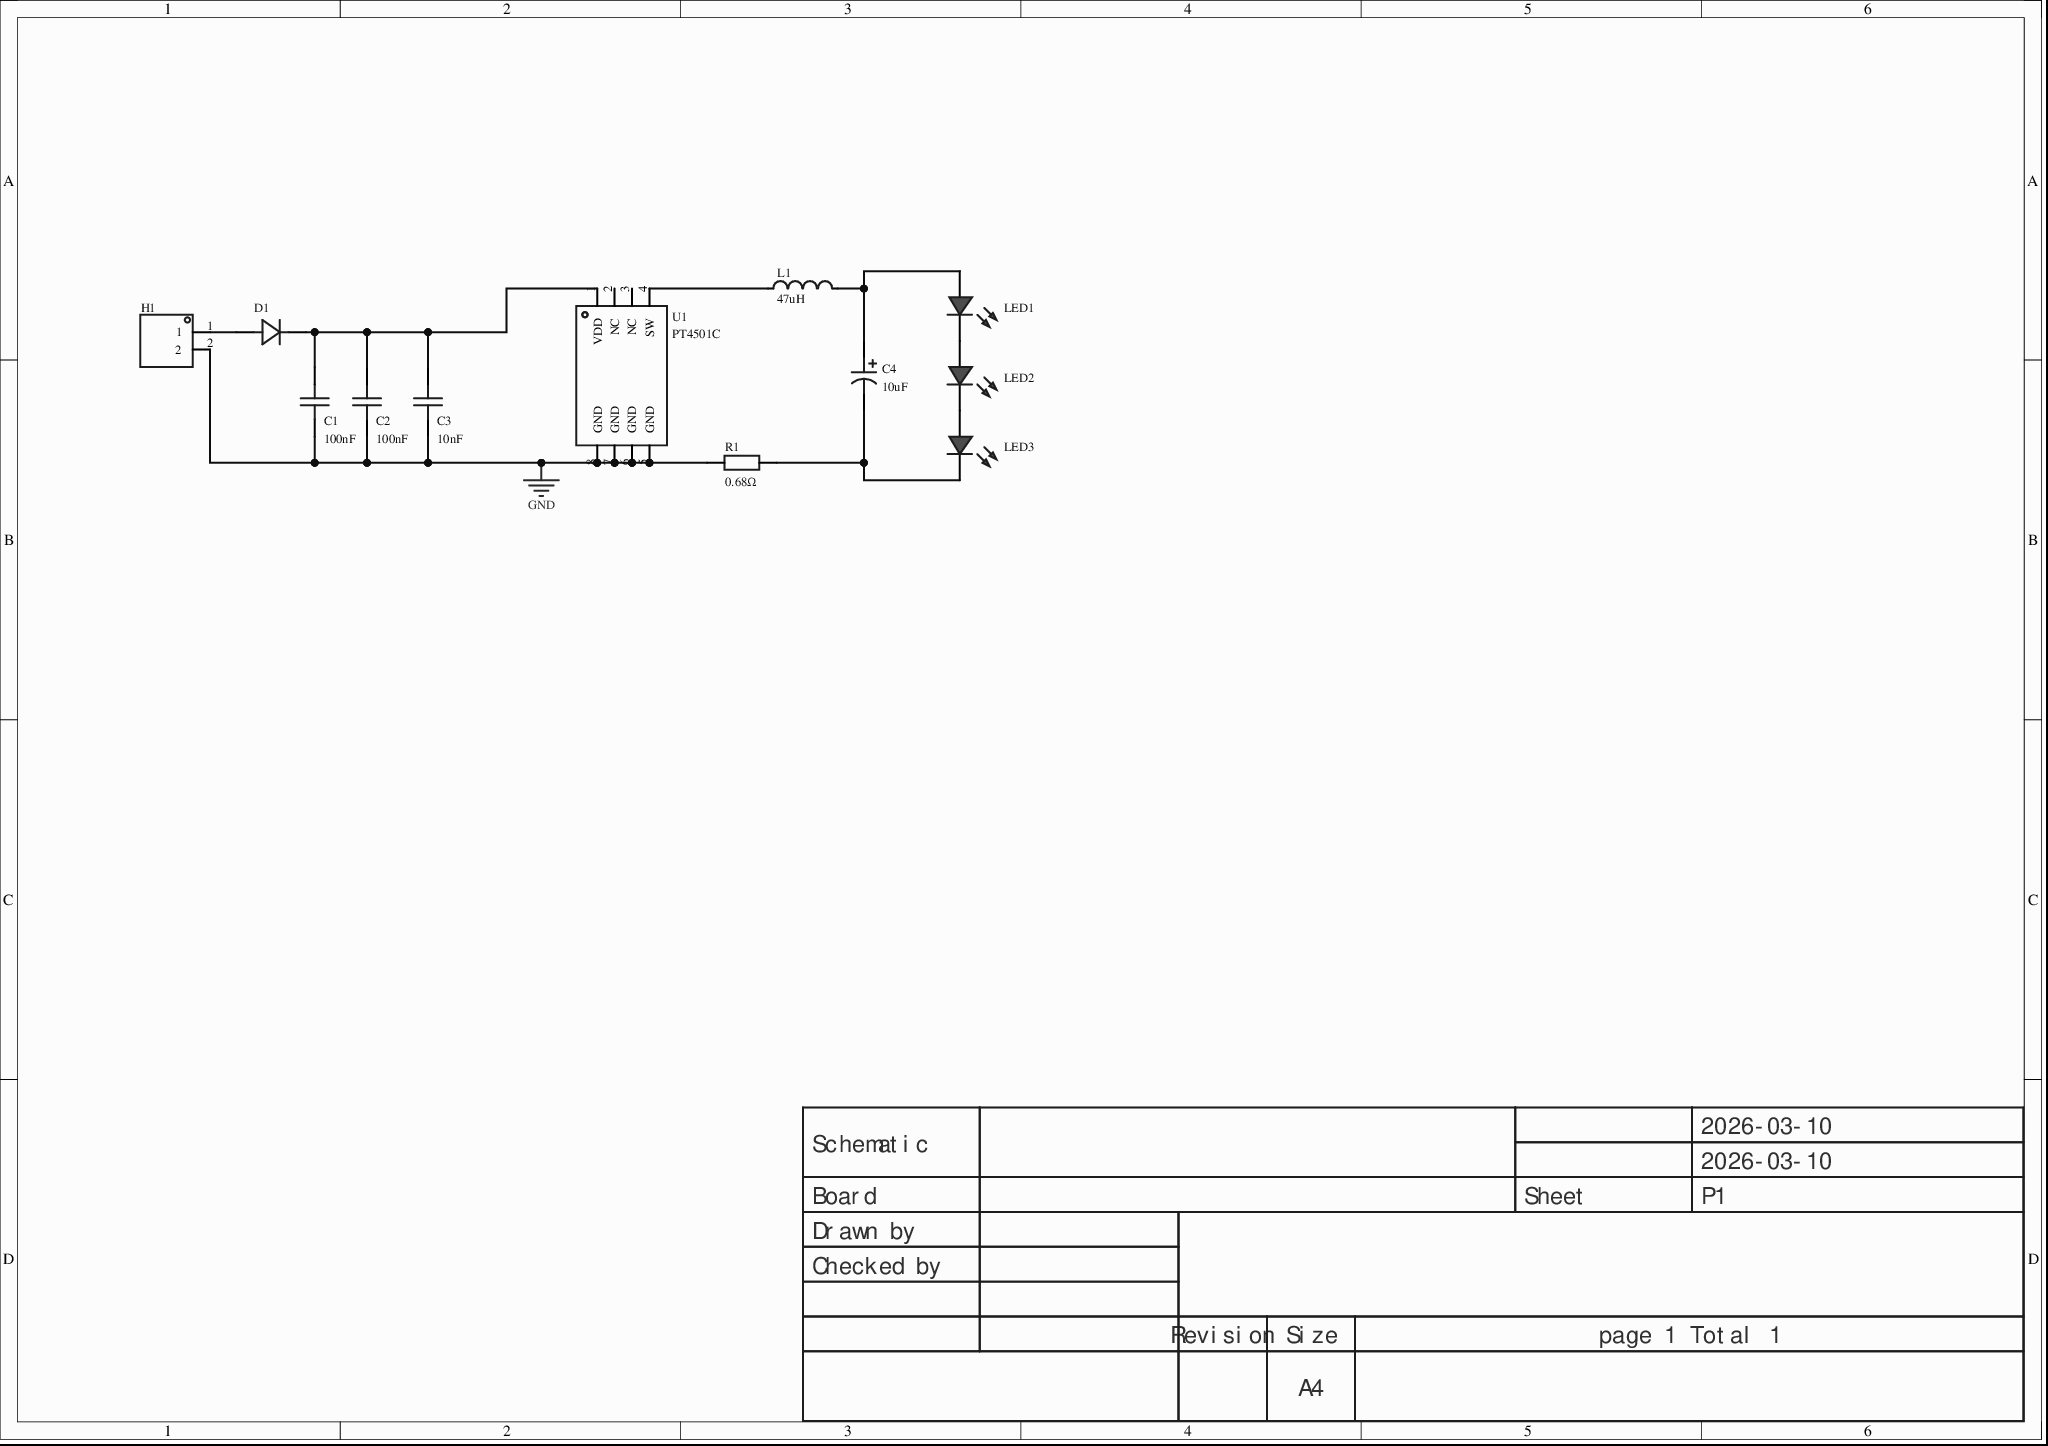
[diagram p0: MISC51773-3.schdoc]
# Altium project MISC51773-2.PrjPcb
1 sheet, 12 parts. Net scope: global (net labels, ports and power ports of the same name join across sheets).
Board file: MISC51773.pcbdoc

## Sheet MISC51773-3.schdoc
size 297 x 209 mm; Version: V1.0; @Project Name: MISC51773; @Update Date: 2026-03-10; @Create Date: 2026-03-10; @Board Name: MISC51773; @Create Time: 23:50:06; @Page Count: 1; @Page No: 1; @Schematic Name: MISC51773; @Update Time: 23:50:06; Size: A4

### Parts
C1  100nF  [CAP-TH_L5.0-W2.5-P5.00-D1.0]
C2  100nF  [CAP-TH_L5.0-W2.5-P5.00-D1.0]
C3  10nF  [CAP-TH_L5.0-W2.5-P5.00-D1.0]
C4  10uF  [CAP-TH_BD5.0-P2.00-D0.8-FD-10UF50VC110GL]
D1  (no value)  [DO_1N4007]
H1  (no value)  [HDR-TH_2P-P2.54-V-M-1]
L1  47uH  [IND-TH_BD7.0-L17.8-P21.80-D0.8]
LED1  (no value)  [LED_TH-3mm]
LED2  (no value)  [LED_TH-3mm]
LED3  (no value)  [LED_TH-3mm]
R1  0.68Ω  [Res_5W]
U1  PT4501C  [SOP-8_L4.9-W3.9-P1.27-LS6.0-BL-EP]

### Nets
GND: C1.2 C2.2 C3.2 H1.2 R1.1 U1.5(GND) U1.6(GND) U1.7(GND) U1.8(GND)
NetC1_1: C1.1 C2.1 C3.1 D1.1(K) U1.1(VDD)
NetC4_1: C4.1 L1.2 LED1.1(C)
NetC4_2: C4.2 LED3.2(A) R1.2
NetD1_2: D1.2(A) H1.1
NetL1_1: L1.1 U1.4(SW)
NetLED1_2: LED1.2(A) LED2.1(C)
NetLED2_2: LED2.2(A) LED3.1(C)

Not connected (* = marked no-connect by the designer): U1 2(NC)* 3(NC)*

### Notes on the sheet
- 2026-03-10
- Schematic
- Board
- Sheet
- P1
- Drawn by
- Checked by
- Revision
- Size
- A4
- page 1 Total 1

### Library data of the parts
C1-C3 = 100nF: Symbol: 100NF_C9900015256; AddInBom: yes; ModelId: 08e3d7481fc7486bb1b263873f51e1e10819f05c4eef4c71ace90d822a990e87; ModelName: CAP-TH_BD5.0-W2.5-P5.08; ModelTransform: 224.652,98.425,0,0,0,0,-0.005,0,-137.795; Device: 100nF; LCSC Part Name: 100nF; SupplierPart: C9900015256; Supplier Footprint: CAP-TH_L5.0-W2.5-P5.00-D1.0; JLCPCB Part Class: Extended Part; Supplier: LCSC; ConvertToPcb: yes; FootprintName: CAP-TH_L5.0-W2.5-P5.00-D1.0
  C1 C2: ManufacturerPart: 100nF
  C3: Manufacturer Part: 10nF
C4 = 10UF50VC110GL: Capacitance: 10uF; Tolerance: ±20%; Rated voltage: 50V; Ripple current: 120mA@100KHz; Equivalent series resistance (ESR): 1.6Ω;; Manufacturer: Econd(米朗电子); AddInBom: yes; Pin Spacing: 2mm; Lifetime: 5000hrs@105℃; Symbol: 10UF50VC110GL; Device: 10UF50VC110GL; LCSC Part Name: 10uF ±20% 50V; SupplierPart: C46867109; ManufacturerPart: 10UF50VC110GL; Supplier Footprint: 插件,D5xL11mm; JLCPCB Part Class: Extended Part; Datasheet: https://item.szlcsc.com/datasheet/10UF50VC110GL/49031974.html; Supplier: LCSC; ConvertToPcb: yes; FootprintName: CAP-TH_BD5.0-P2.00-D0.8-FD-10UF50VC110GL; Value: 10uF; Voltage Rating: 50V; Ripple Current: 120mA@100KHz; Equivalent Series Resistance(ESR): 1.6Ω; Diameter: 5mm; Height - Seated (Max): 11mm; Operating Temperature: -40℃~+105℃
D1 = D_1N4007A: AddInBom: yes; ModelId: 6de1e9b71a0d4751b4e9df530304c1a30819f05c4eef4c71ace90d822a990e87; ModelName: DO-41_D2.4-L4.7-P8.70; ModelTransform: 373.9,94.4,232.29,0,0,0,0,0,-140; Symbol: D_1N4007; Device: D_1N4007A; Supplier Footprint: DO-41; ConvertToPcb: yes; FootprintName: DO_1N4007
H1 = HDR-M_2.54_1x2P: Symbol: 210S-1*2P L=11.6MMGold-plated black; ConvertToPcb: yes; ModelId: 79b2e9f2d70a4d68a1b7098f27c6d4c50819f05c4eef4c71ace90d822a990e87; ModelName: HDR-M-2.54_1x2; ModelTransform: 200,100,0,0,0,0,0,0,-118.11; Device: HDR-M_2.54_1x2P; AddInBom: yes; SupplierPart: C124375; Supplier Footprint: 插件; FootprintName: HDR-TH_2P-P2.54-V-M-1
L1 = IHD1RR470L: Inductance: 47uH; Tolerance: ±15%; Rated current: 1.6A; Saturation current (Isat): -; Type: -; Quality factor: -;; Manufacturer: VISHAY(威世); AddInBom: yes; DC Resistance(DCR): 104mΩ; Symbol: IHD1RR470L; Device: IHD1RR470L; LCSC Part Name: IHD1RR470L; SupplierPart: C1335754; ManufacturerPart: IHD1RR470L; Supplier Footprint: 插件,D6.85xL17.78mm; JLCPCB Part Class: Extended Part; Datasheet: https://item.szlcsc.com/datasheet/IHD1RR470L/1426033.html; Supplier: LCSC; ConvertToPcb: yes; FootprintName: IND-TH_BD7.0-L17.8-P21.80-D0.8; Value: 47uH; Current Rating: 1.6A; Current - Saturation(Isat): -; Q @ Frequency: -; Frequency - Self Resonant: -; Ratings: -
LED1-LED3 = LED_TH-R_3mm: ConvertToPcb: yes; ModelId: a497c992633541038a38947cdc58012f0819f05c4eef4c71ace90d822a990e87; ModelName: LED-TH-3mm_R; ModelTransform: 141.274,153.327,0,0,0,0,-5.984,0,-137.795; Symbol: LED_TH-R; Device: LED_TH-R_3mm; AddInBom: yes; FootprintName: LED_TH-3mm; Supplier Footprint: 插件
R1 = Res_AXIAL-5W: Symbol: Resistor; AddInBom: yes; ModelId: 62c5492292db49eb8544b9c1217b9ea30819f05c4eef4c71ace90d822a990e87; ModelName: RES-TH_BD8.0-L24.5-P29.00; ModelTransform: 1181.1,315.75,453.15,0,0,0,0,0,-120; Device: Res_AXIAL-5W; Value: 0.68Ω; Supplier Footprint: 轴向引线; ConvertToPcb: yes; FootprintName: Res_5W
U1 = PT4516EESH: Dual-channel single-stage linear LED driver IC; Manufacturer: PowTech(华润矽威); AddInBom: yes; ModelId: 94c97984fe8342edbe821bc2ce85d11e0819f05c4eef4c71ace90d822a990e87; ModelName: SOP-8_L4.9-W3.9-H1.7-LS6.0-P1.30; ModelTransform: 236.22,839.658,0,90,0,0,0.0005,-0.0005,0; Symbol: PT4516EESH; Device: PT4516EESH; Manufacturer Part: PT4501C; LCSC Part Name: PT4516EESH 停产; SupplierPart: C126166; Supplier Footprint: SOP-8-EP; JLCPCB Part Class: Extended Part; Datasheet: https://atta.szlcsc.com/upload/public/pdf/source/20170818/C126166_1503051230151895237.pdf; Supplier: LCSC; ConvertToPcb: yes; FootprintName: SOP-8_L4.9-W3.9-P1.27-LS6.0-BL-EP